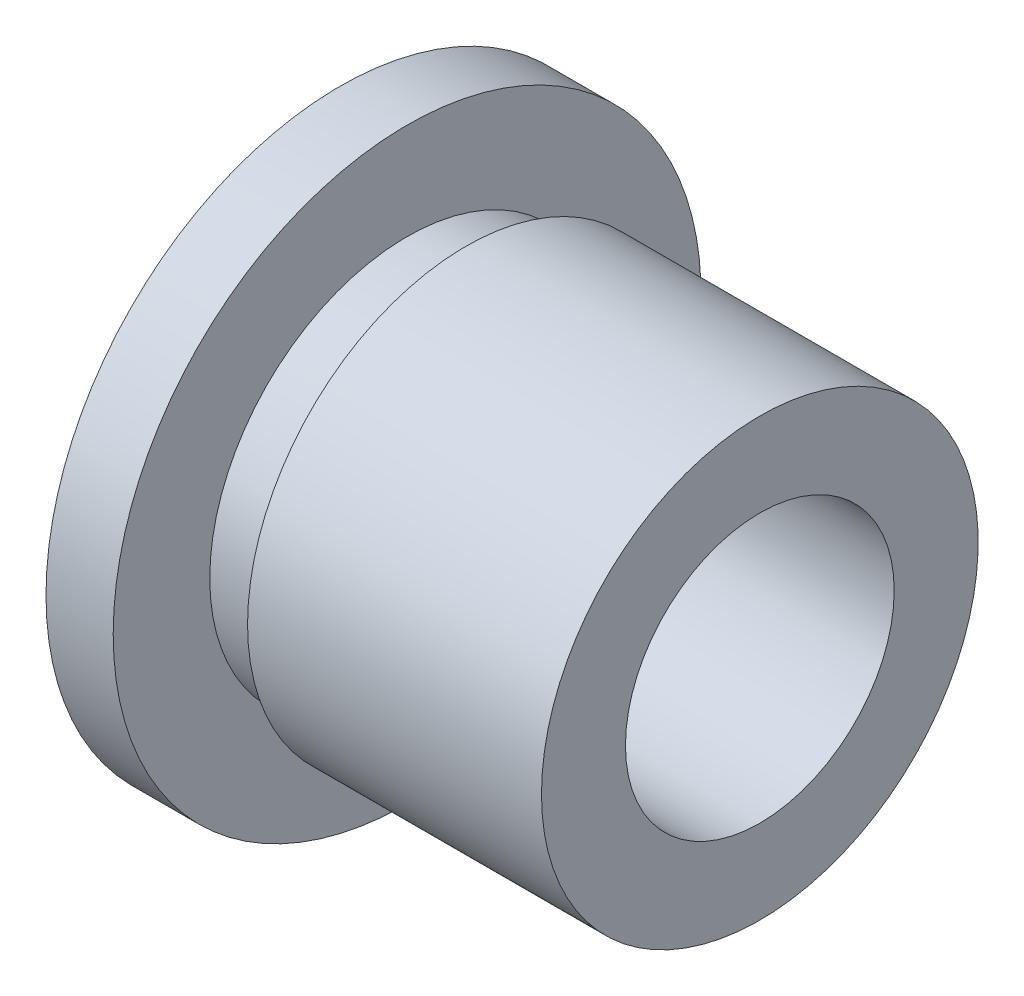
from build123d import *

# Parameters (mm, degrees)
CIRPATTERN1_COUNT = 4


with BuildPart() as part:
    # Sketch1 → Revolve1 (revolve)
    with BuildSketch(Plane.XY, mode=Mode.PRIVATE) as revolve1_sk:
        Polygon((0, 16), (0, 35), (8, 35), (8, 23.5), (15, 23.5), (15, 26), (50, 26), (50, 16), align=None)
    revolve(revolve1_sk.sketch.rotate(Axis((0, 0, 0), (1, 0, 0)), 90), axis=Axis((0, 0, 0), (1, 0, 0)))

    # Sketch3 → Ø10.0 (10) Diameter Hole1 (revolve, cut)
    with BuildSketch(Plane.ZX.offset(25)):
        Polygon((0, 0), (0, 7.004303095), (5, 4), (5, 0), align=None)
    f_10_0_10_diameter_hole1 = revolve(axis=Axis((-6.35, 25, 0), (1, 0, 0)), mode=Mode.SUBTRACT)

    # CirPattern1: Ø10.0 (10) Diameter Hole1 ×4 about axis
    cirpattern1_axis = Axis((0, 0, 0), (1, 0, 0))
    for i in range(1, CIRPATTERN1_COUNT):
        add(f_10_0_10_diameter_hole1.rotate(cirpattern1_axis, i * 360 / CIRPATTERN1_COUNT), mode=Mode.SUBTRACT)


solid = part.part
